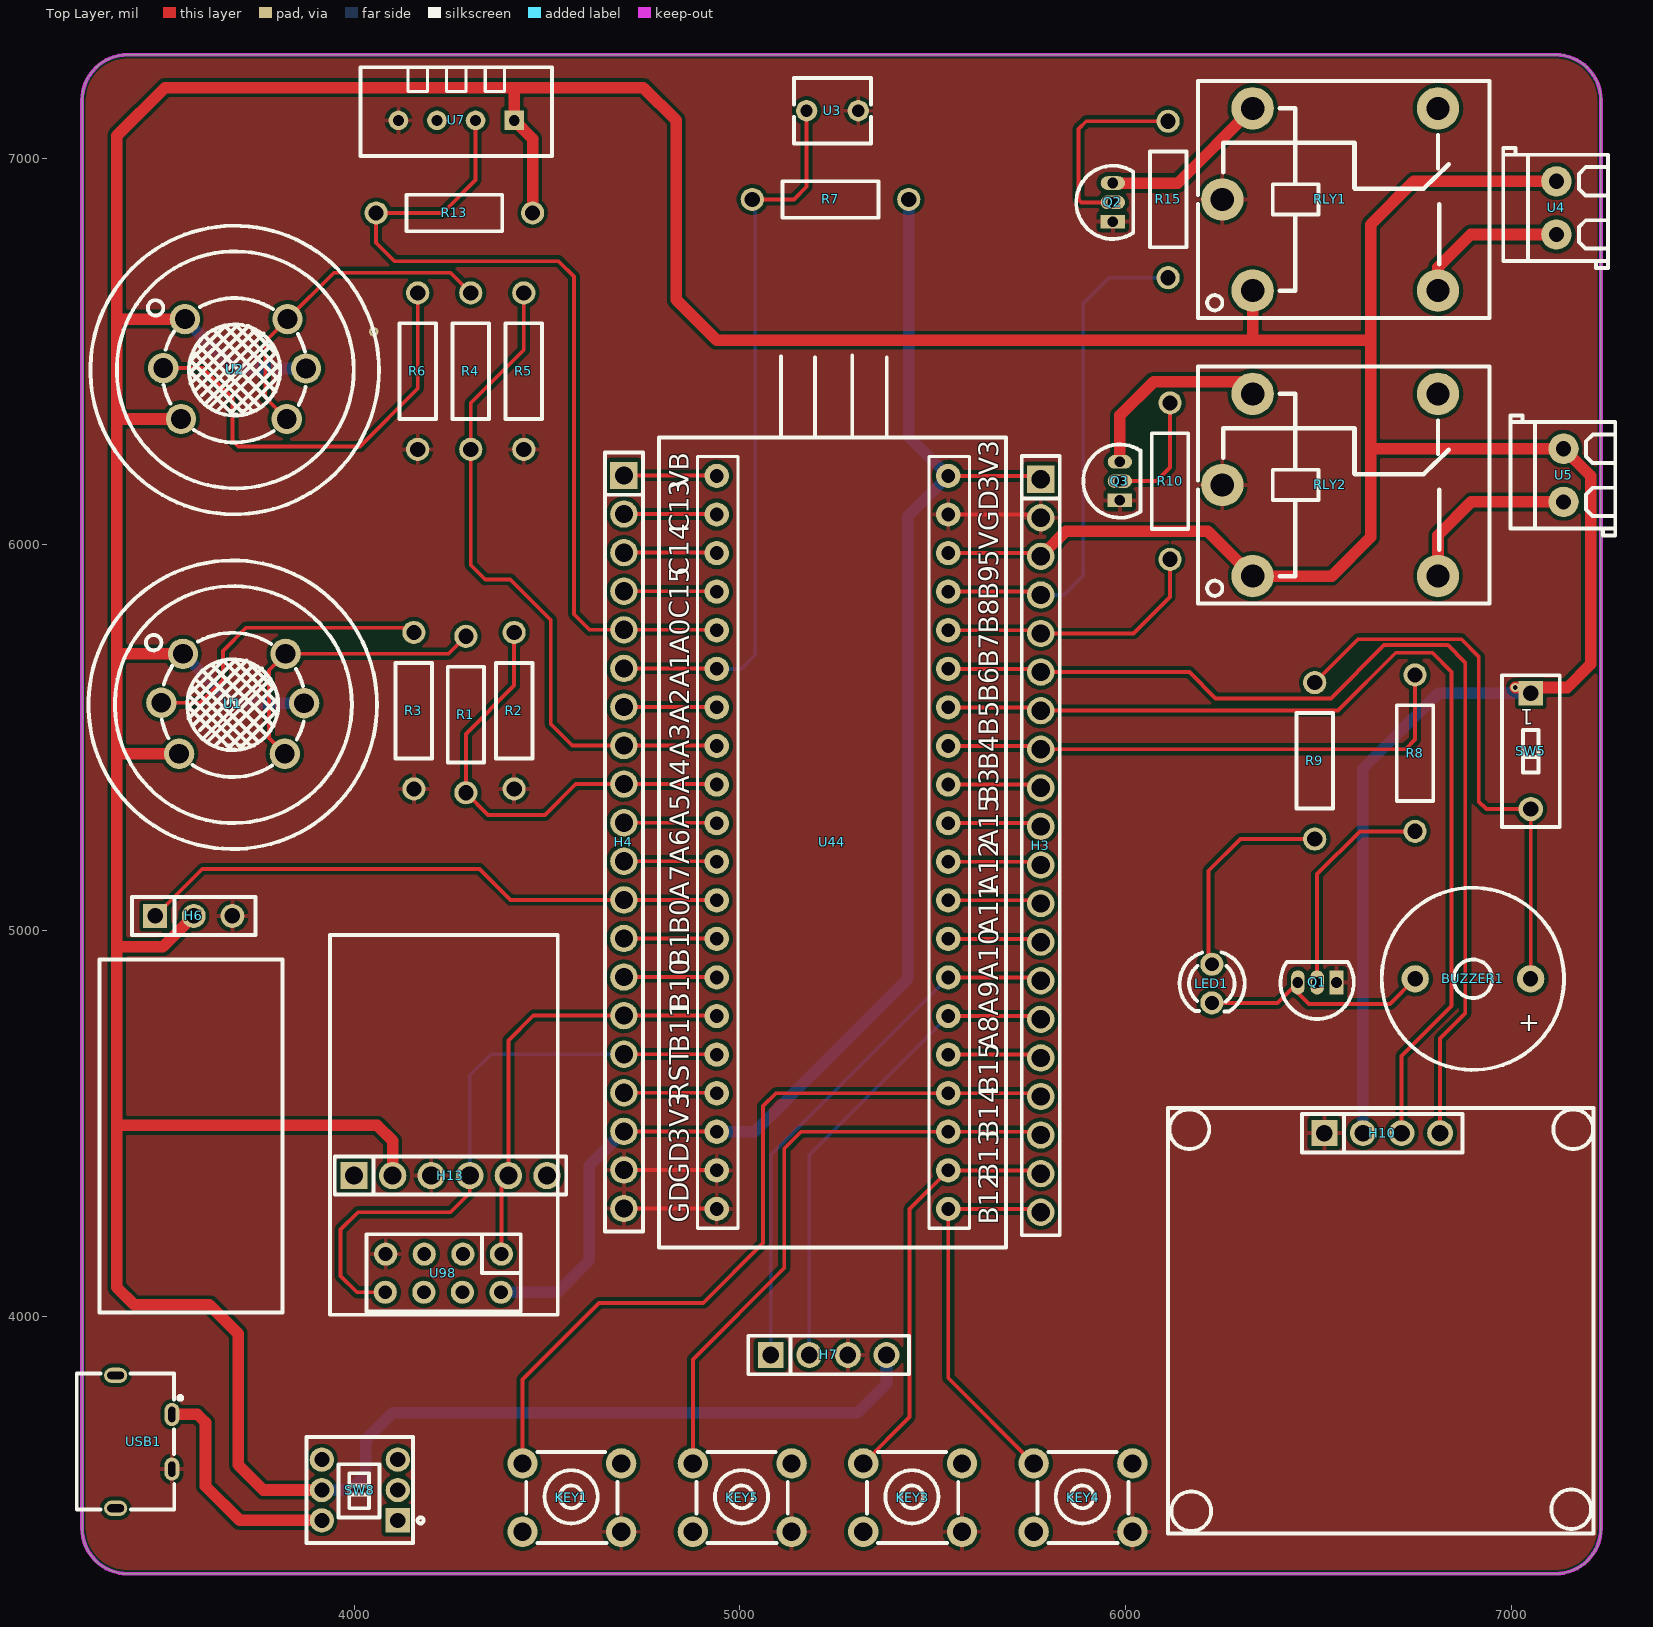
[diagram p0: Top Layer view]
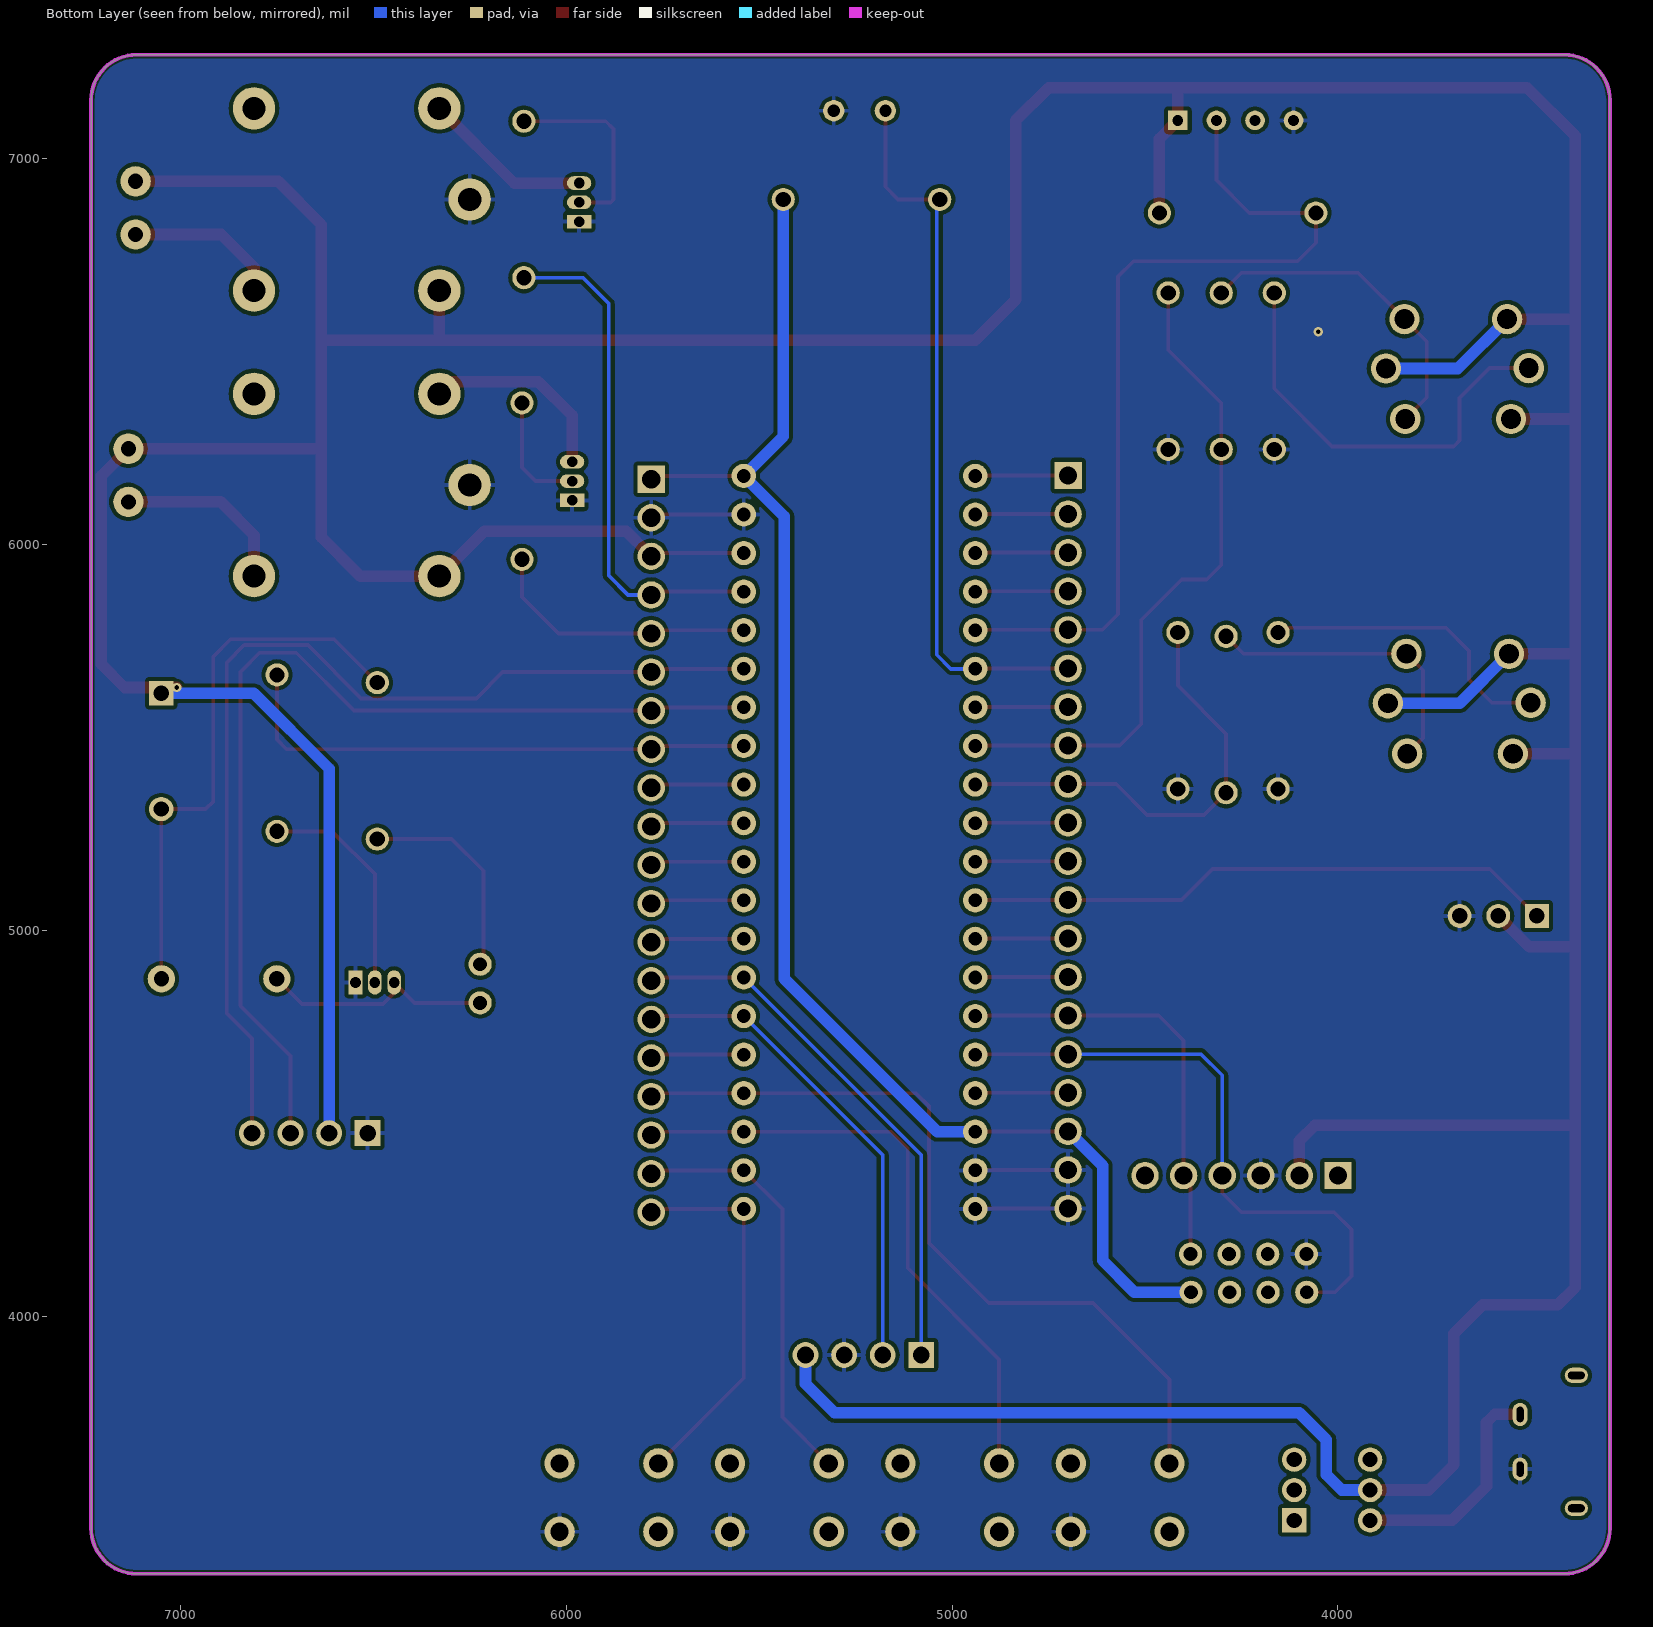
[diagram p1: Bottom Layer view, seen from below]
# Altium PCB MISC52121.pcbdoc
Units mil, origin at the board's own origin, x right, y up, seen from the top; angles counter-clockwise.
Board outline 3937.01 x 3937.01 mil, 2 copper layers (Top Layer, Bottom Layer), stack 62.206 mil thick; 40 components, 52 nets, 202 pads, 2 vias.

## Layer stack, top to bottom
Top Solder Mask Layer: solder mask 0.394, Dk 3.3
Top Layer: signal copper 1.379
Dielectric1: surface 59.449, FR4, Dk 4.5
Bottom Layer: signal copper 1.378
Bottom Solder Mask Layer: solder mask 0.394, Dk 3.3

## Board outline
3413.11,7270 ccw(c3413.11,7151.89) 3295,7151.89 3295,3451.1 ccw(c3413.11,3451.1) 3413.11,3332.99 7113.9,3332.99 ccw(c7113.9,3451.1) 7232.01,3451.1 7232.01,7151.89 ccw(c7113.9,7151.89) 7113.9,7270

## Design rules (kind name [scope] priority, off if disabled: settings)
BoardOutlineClearance copperThickness2oz_1 [All] p2 off: genericclearance=7.99 ignorepadtopadclearanceinfootprint=FALSE except(0: Arc-SplitContinuation Track-SplitContinuation SMDPad-SplitContinuation THPad-SplitContinuation Via-SplitContinuation Fill-SplitContinuation Region-SplitContinuation Poly-SplitContinuation Text-SplitContinuation Hole-SplitContinuation; 5.98: Arc-CutoutEdge SMDPad-CutoutEdge THPad-CutoutEdge Via-CutoutEdge Fill-CutoutEdge Region-CutoutEdge Text-CutoutEdge; 6.93: Hole-OutlineEdge Hole-CutoutEdge; 10: Poly-OutlineEdge Poly-CutoutEdge; 11.81: Arc-OutlineEdge Track-OutlineEdge SMDPad-OutlineEdge THPad-OutlineEdge Via-OutlineEdge Fill-OutlineEdge Region-OutlineEdge Text-OutlineEdge Track-CutoutEdge)
BoardOutlineClearance copperThickness1oz_1 [All] p4: genericclearance=4.02 ignorepadtopadclearanceinfootprint=FALSE except(0: Arc-SplitContinuation Track-SplitContinuation SMDPad-SplitContinuation THPad-SplitContinuation Via-SplitContinuation Fill-SplitContinuation Region-SplitContinuation Poly-SplitContinuation Text-SplitContinuation Hole-SplitContinuation; 6: SMDPad-CutoutEdge THPad-CutoutEdge Via-CutoutEdge Fill-CutoutEdge Region-CutoutEdge Text-CutoutEdge; 6.93: Hole-OutlineEdge Hole-CutoutEdge; 10: Poly-OutlineEdge Poly-CutoutEdge; 11.8: Arc-OutlineEdge Track-OutlineEdge SMDPad-OutlineEdge THPad-OutlineEdge Via-OutlineEdge Fill-OutlineEdge Region-OutlineEdge Text-OutlineEdge; 11.81: Arc-CutoutEdge Track-CutoutEdge)
Clearance copperThickness2oz [All] p1 off: gap=7.99 ignorepadtopadclearanceinfootprint=FALSE except(5.98: SMDPad-Track SMDPad-SMDPad THPad-Track SMDPad-THPad THPad-THPad Track-Via SMDPad-Via THPad-Via Via-Via Fill-Track Region-Track Fill-SMDPad Region-SMDPad Fill-THPad Region-THPad Fill-Via Region-Via Fill-Fill Fill-Region Region-Region Arc-Track Arc-SMDPad Arc-THPad Arc-Via Fill-Arc Region-Arc Arc-Arc Text-Track SMDPad-Text Text-THPad Text-Via Fill-Text Region-Text Arc-Text Text-Text; 6.93: Hole-Track Hole-SMDPad Hole-THPad Hole-Via Fill-Hole Region-Hole Hole-Arc Hole-Text; 10: Poly-Track Poly-SMDPad Poly-THPad Poly-Via Poly-Fill Poly-Region Poly-Poly Poly-Arc Poly-Text Poly-Hole)
Clearance copperThickness1oz [All] p3: gap=4.02 ignorepadtopadclearanceinfootprint=FALSE except(5.98: SMDPad-Track SMDPad-SMDPad THPad-Track SMDPad-THPad THPad-THPad Track-Via SMDPad-Via THPad-Via Via-Via Fill-Track Region-Track Fill-SMDPad Region-SMDPad Fill-THPad Region-THPad Fill-Via Region-Via Fill-Fill Fill-Region Region-Region; 6: Arc-Track Arc-SMDPad Arc-THPad Arc-Via Fill-Arc Region-Arc Arc-Arc Text-Track SMDPad-Text Text-THPad Text-Via Fill-Text Region-Text Arc-Text Text-Text; 6.93: Hole-Track Hole-SMDPad Hole-THPad Hole-Via Fill-Hole Region-Hole Hole-Arc Hole-Text; 10: Poly-Track Poly-SMDPad Poly-THPad Poly-Via Poly-Fill Poly-Region Poly-Poly Poly-Arc Poly-Text Poly-Hole)
Creepage creepage [All] p1: checkdistance=0 ignoreinternallayers=TRUE applytopolygonpour=TRUE
DiffPairsRouting differentialPair [All] p1: maxlimit=6 minlimit=6 mostfreqgap=6 toplayer_minwidth=5 toplayer_prefwidth=10 toplayer_maxwidth=100 toplayer_mingap=6 toplayer_prefgap=6 toplayer_maxgap=6 bottomlayer_minwidth=5 bottomlayer_prefwidth=10 bottomlayer_maxwidth=100 bottomlayer_mingap=6 bottomlayer_prefgap=6 bottomlayer_maxgap=6 maxuncoupledlength=10
HoleToHoleClearance otherClearance [All] p1: gap=11.81 allowstackedmicrovias=TRUE
Length netLength [All] p1: minlimit=0 maxlimit=0
MatchedLengths netLengthTolerance [All] p1: tolerance=1000
PasteMaskExpansion pasteMaskExpansion [All] p1: expansion=0
PlaneConnect innerPlane [All] p1: planeconnectstyle=Relief reliefexpansion=20 reliefentries=4 reliefconductorwidth=10 reliefairgap=10
PolygonConnect copperRegion [All] p1: connectstyle=Relief reliefconductorwidth=10 reliefentries=4 polygonreliefangle="90 Angle" airgapwidth=10 via.connectstyle=Relief via.reliefconductorwidth=10 via.reliefentries=4 via.polygonreliefangle="90 Angle" via.airgapwidth=10
RoutingVias viaSize [All] p1: holewidth=12.01 width=24.02 viastyle="Through Hole" minholewidth=11.81 minwidth=19.68 maxholewidth=248.03 maxwidth=393.7
SolderMaskExpansion solderMaskExpansion [IsVia] p1: expansion=-1000 istentingtop=TRUE
SolderMaskExpansion solderMaskExpansion [All] p2: expansion=2 istentingtop=FALSE
Width copperThickness2oz_2 [All] p1 off: maxlimit=100 minlimit=8 preferedwidth=10
Width copperThickness1oz_2 [All] p2: maxlimit=100 minlimit=5 preferedwidth=10

## Components (designator, comment, footprint, x,y, rotation, side; value= is the part's Value field where it differs from the comment)
BUZZER1 "2.3kHz" BUZ-TH_BD12.0-P7.60-D0.6-FD 6900,4875 r180 top
H3 "" HDR-TH_20P-P2.54-V-F 5780,5220 r270 top
H4 "" HDR-TH_20P-P2.54-V-F 4699.46,5229.58 r270 top
H6 "" HDR-TH_3P-P2.54-V-F 3584.58,5037.88 r0 top
H7 "" HDR-TH_4P-P2.54-V-F 5230,3900 r0 top
H10 "2.54-1*4P female" HDR-TH_4P-P2.54-V-F 6665,4475 r0 top
H13 "" HDR-TH_6P-P2.54-V-M-1 4250,4365 r0 top
KEY1 "Button 1" KEY-TH_4P-L6.0-W6.0-P4.50-LS7.5 4564.46,3530.41 r0 top
KEY3 "Button 2" KEY-TH_4P-L6.0-W6.0-P4.50-LS7.5 5447.8,3530.41 r0 top
KEY4 "Button 4" KEY-TH_4P-L6.0-W6.0-P4.50-LS7.5 5889.46,3530.41 r0 top
KEY5 "Button 5" KEY-TH_4P-L6.0-W6.0-P4.50-LS7.5 5006.13,3530.41 r0 top
LED1 "" LED_TH-3mm 6223.5,4862.73 r270 top
Q1 "" S8050_TO_92 6496.32,4865.58 r180 top
Q2 "" S8050_TO_92 5966.77,6887.54 r90 top
Q3 "" S8050_TO_92 5985,6165 r90 top
R1 "10kΩ" Res_1/4W 4290,5560 r90 top
R2 "10kΩ" Res_1/4W 4415,5570 r90 top
R3 "5Ω" Res_1/4W 4155,5570 r90 top
R4 "10kΩ" Res_1/4W 4302.5,6450 r90 top
R5 "10kΩ" Res_1/4W 4440,6450 r90 top
R6 "5Ω" Res_1/4W 4165,6450 r90 top
R7 "1kΩ" Res_1/4W 5235,6895 r180 top
R8 "1kΩ" Res_1/4W 6750,5460 r270 top
R9 "120" Res_1/4W 6490,5440 r270 top
R10 "1kΩ" Res_1/4W 6115,6165 r90 top
R13 "10kΩ" Res_1/4W 4260,6860 r0 top
R15 "1kΩ" Res_1/4W 6110,6895 r90 top
RLY1 "SRD-05VDC-SL-C" RELAY-TH_SRD-XXVDC-XL-C 6530,6895 r0 top
RLY2 "SRD-05VDC-SL-C" RELAY-TH_SRD-XXVDC-XL-C 6530,6155 r0 top
SW5 "NDS-01V" SW-TH_2P-L3.9-W9.9-P2.54-LS7.6 7050,5465 r270 top
SW8 "TK-6700-1" SW-TH_TK-6700-1 4015,3550 r90 top
U1 "MQ-2" SENSOR-TH_MQ-2 3685.58,5587.88 r0 top
U2 "MQ-5" SENSOR-TH_MQ-2 3690.58,6455.41 r0 top
U3 "光敏电阻-5MM" RES-TH_L4.9-W4.3-P3.4 5240,7125 r180 top
U4 "KF350-3.5-2P" CONN-TH_P3.50_KF350-3.5-2P 7116.51,6873.11 r90 top
U5 "KF350-3.5-2P" CONN-TH_P3.50_KF350-3.5-2P 7135,6180 r90 top
U7 "DHT11" SENSOR-TH_DHT11 4265,7100 r180 top
U44 "" STM32最小系统板 5280,5485 r0 top
U98 "" WiFi封装 4230,4370 r0 top
USB1 "KH-TYPE-C-2P" USB-SMD_KH-TYPE-C-2P 3455,3675 r270 top

## Footprints (in the part's own frame and the unit in brackets; to place one, negate y for a bottom-side part, rotate by r counter-clockwise, add the part's x,y. Pads: shape width x height; smd on the part's side, far side on the other; paste and mask are expansions set on the pad)
BUZ-TH_BD12.0-P7.60-D0.6-FD [mm]
  round 1.8 hole 1 paste+0 mask+0.051: 1(-3.8,0) 2(3.8,0)
  silkscreen extent -6,-6 6,6
CONN-TH_P3.50_KF350-3.5-2P [mm]
  round 2 hole 1: 1(-1.75,0) 2(1.75,0)
  silkscreen extent -3.95,-3.4 3.95,3.5
HDR-TH_3P-P2.54-V-F [mil]
  rect 62x62 hole 40.16: 1(-100,0)
  round 62 hole 40.16: 2(0,0) 3(100,0)
  silkscreen extent -160,-49 160,49
HDR-TH_4P-P2.54-V-F [mm]
  rect 1.7x1.7 hole 1.1: 1(-3.81,0)
  round 1.7 hole 1.1: 2(-1.27,0) 3(1.27,0) 4(3.81,0)
  silkscreen extent -5.29,-1.27 5.29,1.27
HDR-TH_6P-P2.54-V-M-1 [mm]
  rect 1.8x1.8 hole 1.2: 1(-6.35,0)
  round 1.8 hole 1.2: 2(-3.81,0) 3(-1.27,0) 4(1.27,0) 5(3.81,0) 6(6.35,0)
  silkscreen extent -7.62,-1.25 7.62,1.25
HDR-TH_20P-P2.54-V-F [mm]
  rect 1.8x1.8 hole 1.2: 1(-24.13,0)
  round 1.8 hole 1.2: 2(-21.59,0) 3(-19.05,0) 4(-16.51,0) 5(-13.97,0) 6(-11.43,0) 7(-8.89,0) 8(-6.35,0) 9(-3.81,0) 10(-1.27,0) 11(1.27,0) 12(3.81,0) 13(6.35,0) 14(8.89,0) 15(11.43,0) 16(13.97,0) 17(16.51,0) 18(19.05,0) 19(21.59,0) 20(24.13,0)
  silkscreen extent -25.65,-1.25 25.65,1.25
KEY-TH_4P-L6.0-W6.0-P4.50-LS7.5 [mm]
  round 2 hole 1.2 paste+0 mask+0.051: 1(-3.25,-2.25) 2(3.25,-2.25) 3(3.25,2.25) 4(-3.25,2.25)
  silkscreen extent -3,-3 3,3
LED_TH-3mm [mil]
  round 60 hole 36 paste+0 mask+2: 1(-50,0) 2(50,0)
  silkscreen extent -81,-84 72,85
RELAY-TH_SRD-XXVDC-XL-C [mil]
  round 110 hole 60: 1(-200.79,-236.22) 2(279.52,-236.2) 3(279.53,236.2) 4(-200.79,236.22) 5(-279.53,0)
  silkscreen extent -342,-307 413,307
RES-TH_L4.9-W4.3-P3.4 [mm]
  round 1.4 hole 0.8 paste+0 mask+0.05: 1(-1.7,0) 2(1.7,0)
  silkscreen extent -2.54,-2.16 2.54,2.16
Res_1/4W [mil]
  round 60 hole 39.37 paste+0 mask+2: 1(-202.76,0) 2(202.76,0)
  silkscreen extent -124,-47 124,47
S8050_TO_92 [mil]
  rect 35.4x63 hole 27.6 paste+0 mask+2: 1(-50,0)
  oval 35.4x63 hole 27.6 paste+0 mask+2: 2(0,0) 3(50,0)
  silkscreen extent -95,-53 95,95
SENSOR-TH_DHT11 [mil]
  rect 51x51 hole 28: 1(-150,0)
  round 51 hole 28: 2(-50,0) 3(50,0) 4(150,0)
  silkscreen extent -248,-138 248,93
SENSOR-TH_MQ-2 [mil]
  round 78.74 hole 51.18: 1(-129,129.5) 2(-185,2.5) 3(-139,-129.5) 4(135,-129.5) 5(185,1.5) 6(137,129.5)
  silkscreen extent -374,-376 374,371
STM32最小系统板 [mm]
  round 1.6 hole 0.9: 1(-8.634,17.614) 2(-8.634,15.074) 3(-8.634,12.534) 4(-8.634,9.994) 5(-8.634,7.454) 6(-8.634,4.914) 7(-8.634,2.374) 8(-8.634,-0.166) 9(-8.634,-2.706) 10(-8.634,-5.246) 11(-8.634,-7.786) 12(-8.634,-10.326) 13(-8.634,-12.866) 14(-8.634,-15.406) 15(-8.634,-17.946) 16(-8.634,-20.486) 17(-8.634,-23.026) 18(-8.634,-25.566) 19(-8.634,-28.106) 20(-8.634,-30.646) 21(6.606,17.614) 22(6.606,15.074) 23(6.606,12.534) 24(6.606,9.994) 25(6.606,7.454) 26(6.606,4.914) 27(6.606,2.374) 28(6.606,-0.166) 29(6.606,-2.706) 30(6.606,-5.246) 31(6.606,-7.786) 32(6.606,-10.326) 33(6.606,-12.866) 34(6.606,-15.406) 35(6.606,-17.946) 36(6.606,-20.486) 37(6.606,-23.026) 38(6.606,-25.566) 39(6.606,-28.106) 40(6.606,-30.646)
  silkscreen extent -12.44,-33.19 10.42,25.54
SW-TH_2P-L3.9-W9.9-P2.54-LS7.6 [mm]
  rect 1.6x1.6 hole 1 paste+0 mask+0.05: 1(-3.81,0)
  round 1.6 hole 1 paste+0 mask+0.05: 2(3.81,0)
  silkscreen extent -5,-1.91 5,1.91
SW-TH_TK-6700-1 [mm]
  rect 1.6x1.6 hole 1 paste+0 mask+0.051: 1(-2,-2.5)
  round 1.6 hole 1 paste+0 mask+0.051: 2(0,-2.5) 3(2,-2.5)
  round 1.6 hole 1 copper offset 0,0 paste+0 mask+0.051: 4(-2,2.5) 5(0,2.5) 6(2,2.5)
  silkscreen extent -3.5,-4.2 3.5,3.5
USB-SMD_KH-TYPE-C-2P [mm]
  oval 1.524x1 hole 0.45 slot 1 at 0 deg paste+0 mask+0.05: 1(-1.8,1.85) 2(1.8,1.85)
  oval 1x1.524 hole 0.5 slot 1.1 at 90 deg paste+0 mask+0.05: 3(4.375,-1.85) 4(-4.375,-1.85)
  silkscreen extent -4.5,-4.41 4.46,2.53
WiFi封装 [mil]
  round 60 hole 36: 1(152.01,-208.54) 2(150.91,-307.4) 3(52.01,-208.54) 4(50.91,-307.4) 5(-47.99,-208.54) 6(-49.09,-307.4) 7(-147.99,-208.54) 8(-149.09,-307.4)
  silkscreen extent -293,-366 298,618

## Via types
v1: diameter 24.02, hole 12, Top Layer to Bottom Layer, 2 vias

## Nets (pads, with @x,y where several pads share a name; then routed paths per layer and width w, separated by ;. In a path a pad name is that pad's centre, name@x,y a point inside that pad or via, vN(x,y) a via of type N, cw(c..) or ccw(c..) an arc to the next point about the centre after c; other vN are vias at no path point)
3V3: H3.1 H4.18 R7.1 U44.18 U44.21 U98.2 | length 3895.4
  Top Layer w10: H4.18 U44.18@4940,4479.58 ; U44.21 H3.1@5795,6178.46
  Bottom Layer w30: U98.2 4527.6,4062.6 4610,4145 4610,4390.12 H4.18 ; U44.18 5038.46,4478.46 5435,4875 5435,6073.39 U44.21 5437.76,6280.78 R7.1
$1N1: LED1.1 R9.2 | length 554.9
  Top Layer w10: LED1.1 6215,4921.24 6215,5155 6297.24,5237.24 R9.2
$1N2: Q2.3 RLY1.4 | length 442.7
  Top Layer w30: Q2.3 6135.53,6937.54 RLY1.4
$1N3: Q3.3 RLY2.4 | length 513.6
  Top Layer w30: Q3.3 5985,6335.21 6072.38,6422.59 6297.84,6422.59 RLY2.4
$1N6: Q2.2 R15.2 | length 515.4
  Top Layer w10: Q2.2 5885,6887.54 5877.93,6894.61 5877.93,7077.93 5897.76,7097.76 R15.2
$1N7: Q3.2 R10.2 | length 312.3
  Top Layer w10: Q3.2 6080,6165 6115,6200 R10.2
$1N17: Q1.2 R8.2 | length 580.4
  Top Layer w10: Q1.2 6496.32,5146.32 6607.24,5257.24 R8.2
$1N29: RLY2.2 U5.1 | length 467.1
  Top Layer w30: RLY2.2 6809.53,6024.53 6896.1,6111.1 U5.1
$1N30: RLY1.2 U4.1 | length 402.8
  Top Layer w30: RLY1.2 6809.53,6719.53 6894.21,6804.21 U4.1
$1N42: BUZZER1.1 R9.1 SW5.2 | length 1448.6
  Top Layer w10: R9.1 6602.24,5755 6870,5755 6915,5710 6915,5335 6935,5315 SW5.2 7050,4875.4 BUZZER1.1
$1N43: BUZZER1.2 LED1.2 Q1.3 | length 614.5
  Top Layer w10: LED1.2 6393.47,4812.73 Q1.3 6446.32,4838.68 6475,4810 6685.4,4810 BUZZER1.2
$1N64: H4.17 U44.17 | length 240.5
  Top Layer w10: H4.17 U44.17@4940,4579.58
$1N67: H4.14 U44.14 | length 240.5
  Top Layer w10: H4.14 U44.14@4940,4879.58
$1N68: H4.13 U44.13 | length 240.5
  Top Layer w10: H4.13 U44.13@4940,4979.58
$1N70: H4.11 U44.11 | length 240.5
  Top Layer w10: H4.11 U44.11@4940,5179.58
$1N74: H4.7 U44.7 | length 240.5
  Top Layer w10: H4.7 U44.7@4940,5579.58
$1N77: H4.4 U44.4 | length 240.5
  Top Layer w10: H4.4 U44.4@4940,5879.58
$1N78: H4.3 U44.3 | length 240.5
  Top Layer w10: H4.3 U44.3@4940,5979.58
$1N79: H4.2 U44.2 | length 240.5
  Top Layer w10: H4.2 U44.2@4940,6079.58
$1N80: H4.1 U44.1 | length 240.5
  Top Layer w10: H4.1 U44.1@4940,6179.58
$1N89: H3.9 U44.29 | length 254.9
  Top Layer w10: U44.29 H3.9@5795,5378.46
$1N90: H3.10 U44.30 | length 254.9
  Top Layer w10: U44.30 H3.10@5795,5278.46
$1N91: H3.11 U44.31 | length 254.9
  Top Layer w10: U44.31 H3.11@5795,5178.46
$1N92: H3.12 U44.32 | length 254.9
  Top Layer w10: U44.32 H3.12@5795,5078.46
$1N93: H3.13 U44.33 | length 254.9
  Top Layer w10: U44.33 H3.13@5795,4978.46
$1N96: H3.16 U44.36 | length 254.9
  Top Layer w10: U44.36 H3.16@5795,4678.46
$1N103: R6.2 U2.2 | length 1117.8
  Top Layer w10: U2.2 3607.09,6457.91 3685,6380 3685,6270 3700,6255 4015,6255 4165,6405 R6.2
$1N104: R3.2 U1.2 | length 784
  Top Layer w10: U1.2 3600.38,5590.38 3660,5650 3660,5725 3720,5785 4142.76,5785 R3.2
$1N107: R4.2 U2.4 U2.6 | length 852.2
  Top Layer w10: U2.4 3770,6381.49 3770,6527.33 U2.6 3947.67,6705 4250.26,6705 R4.2
$1N108: R1.2 U1.4 U1.6 | length 779.7
  Top Layer w10: U1.4 3780,5498.95 3780,5674.8 U1.6 4244.61,5717.38 R1.2
+5V: H3.3 H6.2 H7.4 H10.2 H13.2 R13.2 RLY1.1 RLY2.1 SW5.1 SW8.5 U1.1 U1.3 U1.5 U2.1 U2.3 U2.5 U4.2 U5.2 U7.1 U44.23 | length 17757.5
  Top Layer w10: U44.23 H3.3@5788.46,5978.46
  Top Layer w30: 3385.03,5717.38 U1.1 ; U1.3 3388.56,5458.38 3385,5461.93 ; U2.3 3388.18,6325.91 3385,6329.09 ; U2.1 3387.29,6584.91 3385,6587.2 ; H6.2 3504.66,4957.95 3385,4957.95 ; SW8.5 3765,3550 3700,3615 3700,3955 3625,4030 3430,4030 3385,4075 3385,4490.1 ; H13.2 4100,4455 4060,4495 3389.9,4495 3385,4490.1 ; R13.2 4462.76,7052.24 U7.1 4415,7183.35 4416.65,7185 ; H3.3 5788.46,5978.46 5845,6035 6212.99,6035 RLY2.1 6533.78,5918.78 6635,6020 6635,6254.11 ; RLY1.1 6329.21,6530.46 6328.75,6530 ; v1(7010,5630) 7145,5630 7205,5690 7205,6178.9 U5.2 6640.22,6248.9 6635,6254.11 ; U4.2 6747,6942 6635,6830 6635,6530 ; 3385,4490.1 3385,4957.95 ; 3385,4957.95 3385,5461.93 ; 3385,5461.93 3385,5717.41 3385,6329.09 ; 3385,6329.09 3385,6587.2 ; 3385,6587.2 3385,7060 3510,7185 4416.65,7185 ; 4416.65,7185 4750,7185 4835,7100 4835,6635 4940,6530 6328.75,6530 ; 6328.75,6530 6635,6530 ; 6635,6254.11 6635,6530
  Bottom Layer w30: U1.1 3684.58,5589.38 U1.5 ; U2.1 3689.58,6456.91 U2.5 ; SW8.5 3990,3550 4030,3590 4030,3680 4100,3750 5305,3750 5380,3825 H7.4 ; H10.2 6615,5420 6810,5615 SW5.1
GND: H3.2 H4.19 H4.20 H6.3 H7.3 H10.1 H13.3 KEY1.2 KEY3.2 KEY4.2 KEY5.2 Q1.1 Q2.1 Q3.1 R2.1 R3.1 R5.1 R6.1 RLY1.5 RLY2.5 U3.1 U7.4 U44.19 U44.20 U44.22 U98.7 USB1.2 | length 736
  Top Layer w10: H4.20 U44.20@4940,4279.58 ; H4.19 U44.19@4940,4379.58 ; U44.22 H3.2@5795,6078.46
  other v1: 4051.2,6552.12
PA0: H4.5 R13.1 U7.2 U44.5 | length 2336.1
  Top Layer w10: U7.2 4315,6945 4230,6860 R13.1 4057.24,6782.76 4105,6735 4530,6735 4570,6695 4570,5820 4610.42,5779.58 H4.5 U44.5@4940,5779.58
PA1: H4.6 R7.2 U3.2 U44.6 | length 1890.3
  Top Layer w10: H4.6 U44.6@4940,5679.58 ; R7.2 5140,6895 5173.07,6928.07 U3.2
  Bottom Layer w10: U44.6 5003.46,5678.46 5040,5715 5040,6887.24 R7.2
PA3: H4.8 R4.1 R5.2 U44.8 | length 1751.7
  Top Layer w10: R5.2 4440,6505 4302.5,6367.5 R4.1 4302.5,5947.5 4340,5910 4405,5910 4510,5805 4510,5535 4565.42,5479.58 H4.8 U44.8@4940,5479.58
PA4: H4.9 R1.1 R2.2 U44.9 | length 1174
  Top Layer w10: R2.2 4415,5635 4290,5510 R1.1 4347.24,5300 4495,5300 4574.58,5379.58 H4.9 U44.9@4940,5379.58
PA5: H4.10 U44.10 | length 240.5
  Top Layer w10: H4.10 U44.10@4940,5279.58
PA7: H4.12 H6.1 U44.12 | length 1539.3
  Top Layer w10: H6.1 3606.7,5160 4325,5160 4405.42,5079.58 H4.12 U44.12@4940,5079.58
PB5: H3.8 R8.1 U44.28 | length 1403
  Top Layer w10: U44.28 H3.8@5795,5478.46 ; H3.8 6725,5470 6750,5495 R8.1
PB6: H3.7 H10.3 U44.27 | length 2651.6
  Top Layer w10: U44.27 H3.7@5795,5578.46 ; H3.7 6550,5570 6700,5720 6795,5720 6845,5670 6845,4805 6715,4675 H10.3
PB7: H3.6 H10.4 U44.26 | length 2706
  Top Layer w10: U44.26 H3.6@5795,5678.46 ; H3.6 6165,5670 6233.22,5601.78 6531.78,5601.78 6670,5740 6835,5740 6880,5695 6880,4785 6815,4720 H10.4
PB8: H3.5 R10.1 U44.25 | length 726.5
  Top Layer w10: U44.25 H3.5@5795,5778.46 ; H3.5 6020,5770 6115,5865 R10.1
PB9: H3.4 R15.1 U44.24 | length 1338.5
  Top Layer w10: U44.24 H3.4@5795,5878.46
  Bottom Layer w10: H3.4 5840,5870 5890,5920 5890,6625 5957.24,6692.24 R15.1
PB12: H3.20 KEY4.4 U44.40 | length 1006.1
  Top Layer w10: KEY4.4 5540.08,3840.43 U44.40 H3.20@5795,4278.46
PB13: H3.19 KEY3.4 U44.39 | length 1105.6
  Top Layer w10: KEY3.4 5440,3739.14 5440,4278.39 U44.39 H3.19@5795,4378.46
PB14: H3.18 KEY5.4 U44.38 | length 1612.1
  Top Layer w10: KEY5.4 4878.18,3888.18 5115,4125 5115,4435 5158.46,4478.46 U44.38 H3.18@5795,4478.46
PB15: H3.17 KEY1.4 U44.37 | length 2091.3
  Top Layer w10: KEY1.4 4436.51,3836.51 4635,4035 4905,4035 5060,4190 5060,4545 5093.46,4578.46 U44.37 H3.17@5795,4578.46
U1_RX: H3.14 H7.1 U44.34 | length 1424
  Top Layer w10: U44.34 H3.14@5795,4878.46
  Bottom Layer w10: H7.1 5080,4418.39 U44.34
U1_TX: H3.15 H7.2 U44.35 | length 1282.5
  Top Layer w10: U44.35 H3.15@5795,4778.46
  Bottom Layer w10: H7.2 5180,4418.39 U44.35
U3_RX: H4.16 H13.4 U44.16 U98.8 | length 1595.4
  Top Layer w10: U98.8 4007.4,4062.6 3965,4105 3965,4225 4010,4270 4250,4270 4300,4320 H13.4 ; H4.16 U44.16@4940,4679.58
  Bottom Layer w10: H13.4 4300,4625 4354.58,4679.58 H4.16
U3_TX: H4.15 H13.5 U44.15 U98.1 | length 1127.7
  Top Layer w10: U98.1 4382.01,4347.01 H13.5 4400,4715 4464.58,4779.58 H4.15 U44.15@4940,4779.58
VUSB: SW8.4 USB1.1 | length 599.1
  Top Layer w30: USB1.1 3594.13,3745.87 3615,3725 3615,3560 3703.74,3471.26 SW8.4
pads on no net: H13.1 H13.6 KEY1.1 KEY1.3 KEY3.1 KEY3.3 KEY4.1 KEY4.3 KEY5.1 KEY5.3 RLY1.3 RLY2.3 SW8.1 SW8.2 SW8.3 SW8.6 U7.3 U98.3 U98.4 U98.5 U98.6 USB1.3 USB1.4

## Polygon pours and split planes (outlines as drawn)
GND on Bottom Layer (solid, remove dead copper, pour order 2): 3000,7550 3000,3000 7640,3000 7640,7550
GND on Top Layer (solid, remove dead copper, pour order 0): 3110,7440 3110,3130 7615,3130 7615,7440

## Keep-outs
Board Outline Layer:
  the board outline again, w10

## Silkscreen, mask and mechanical layers (free items; w line width, h text height)
Top Silkscreen Layer:
  lines w10: 3340,4010 3340,4925 3815,4925 3815,4010 3340,4010